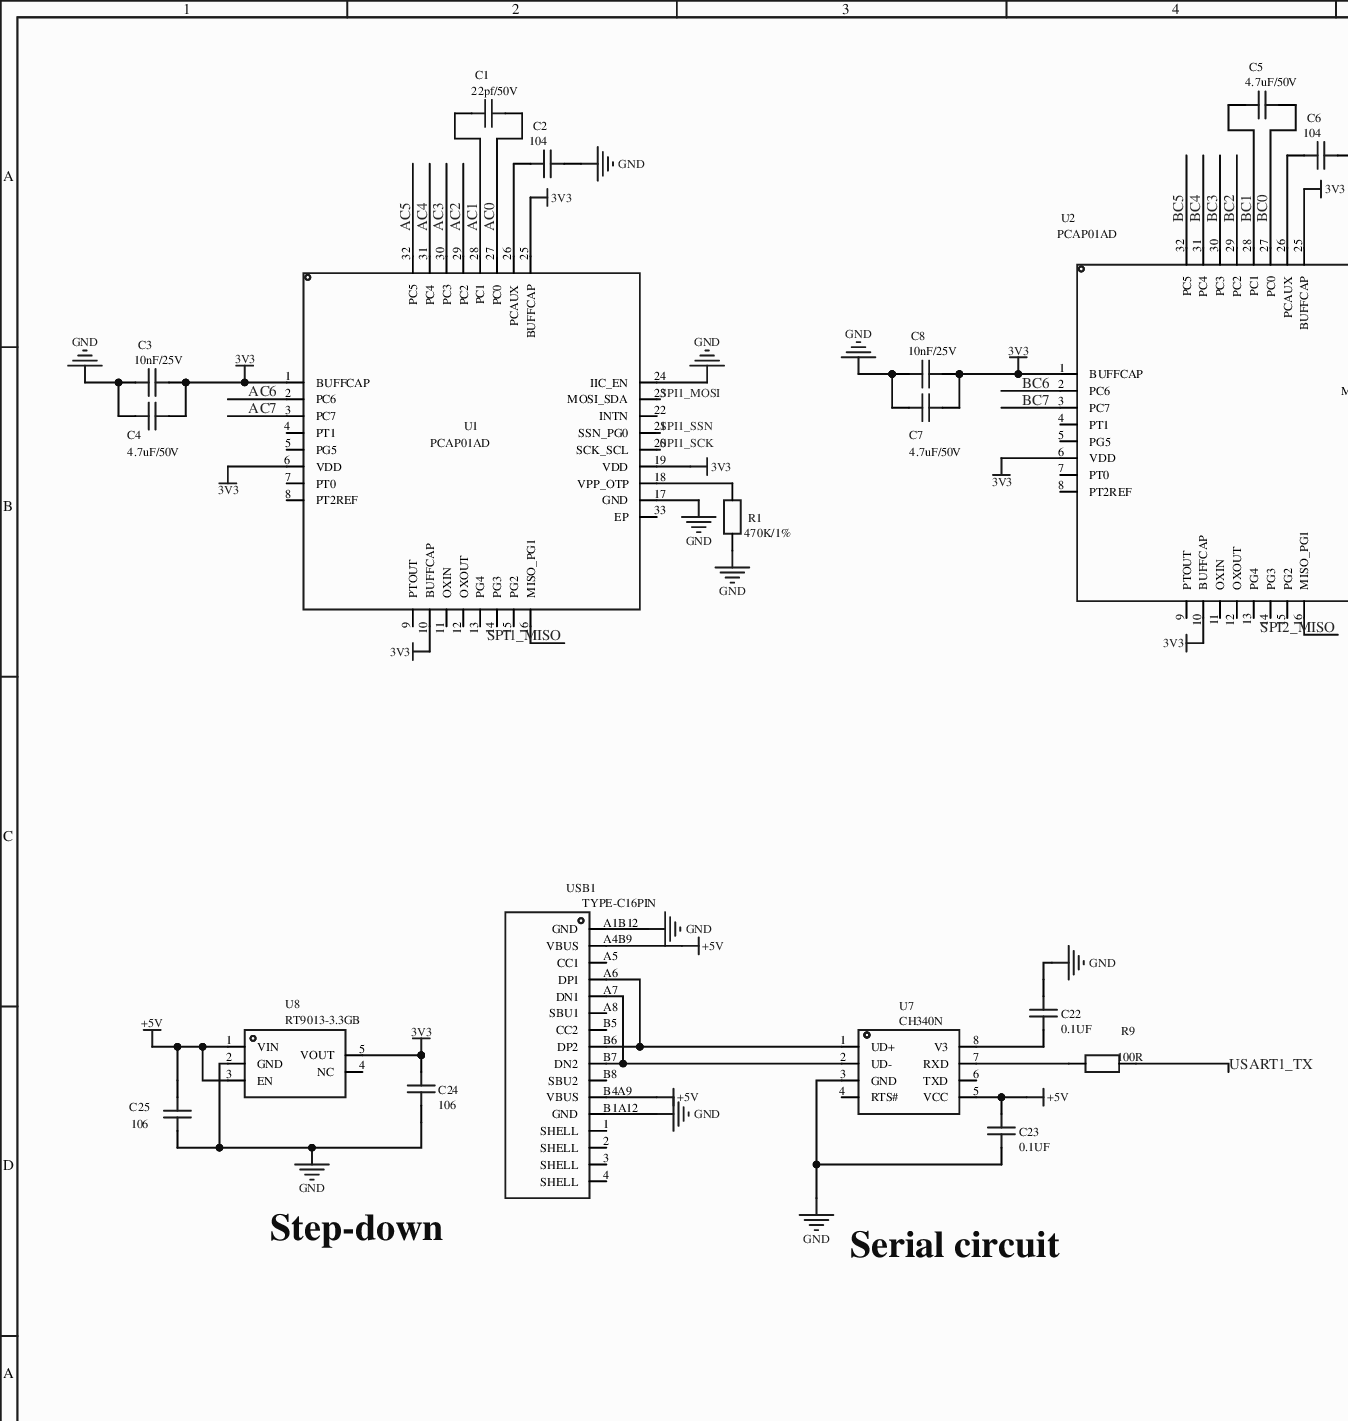
[diagram p0: MISC49858-3.schdoc, top left]
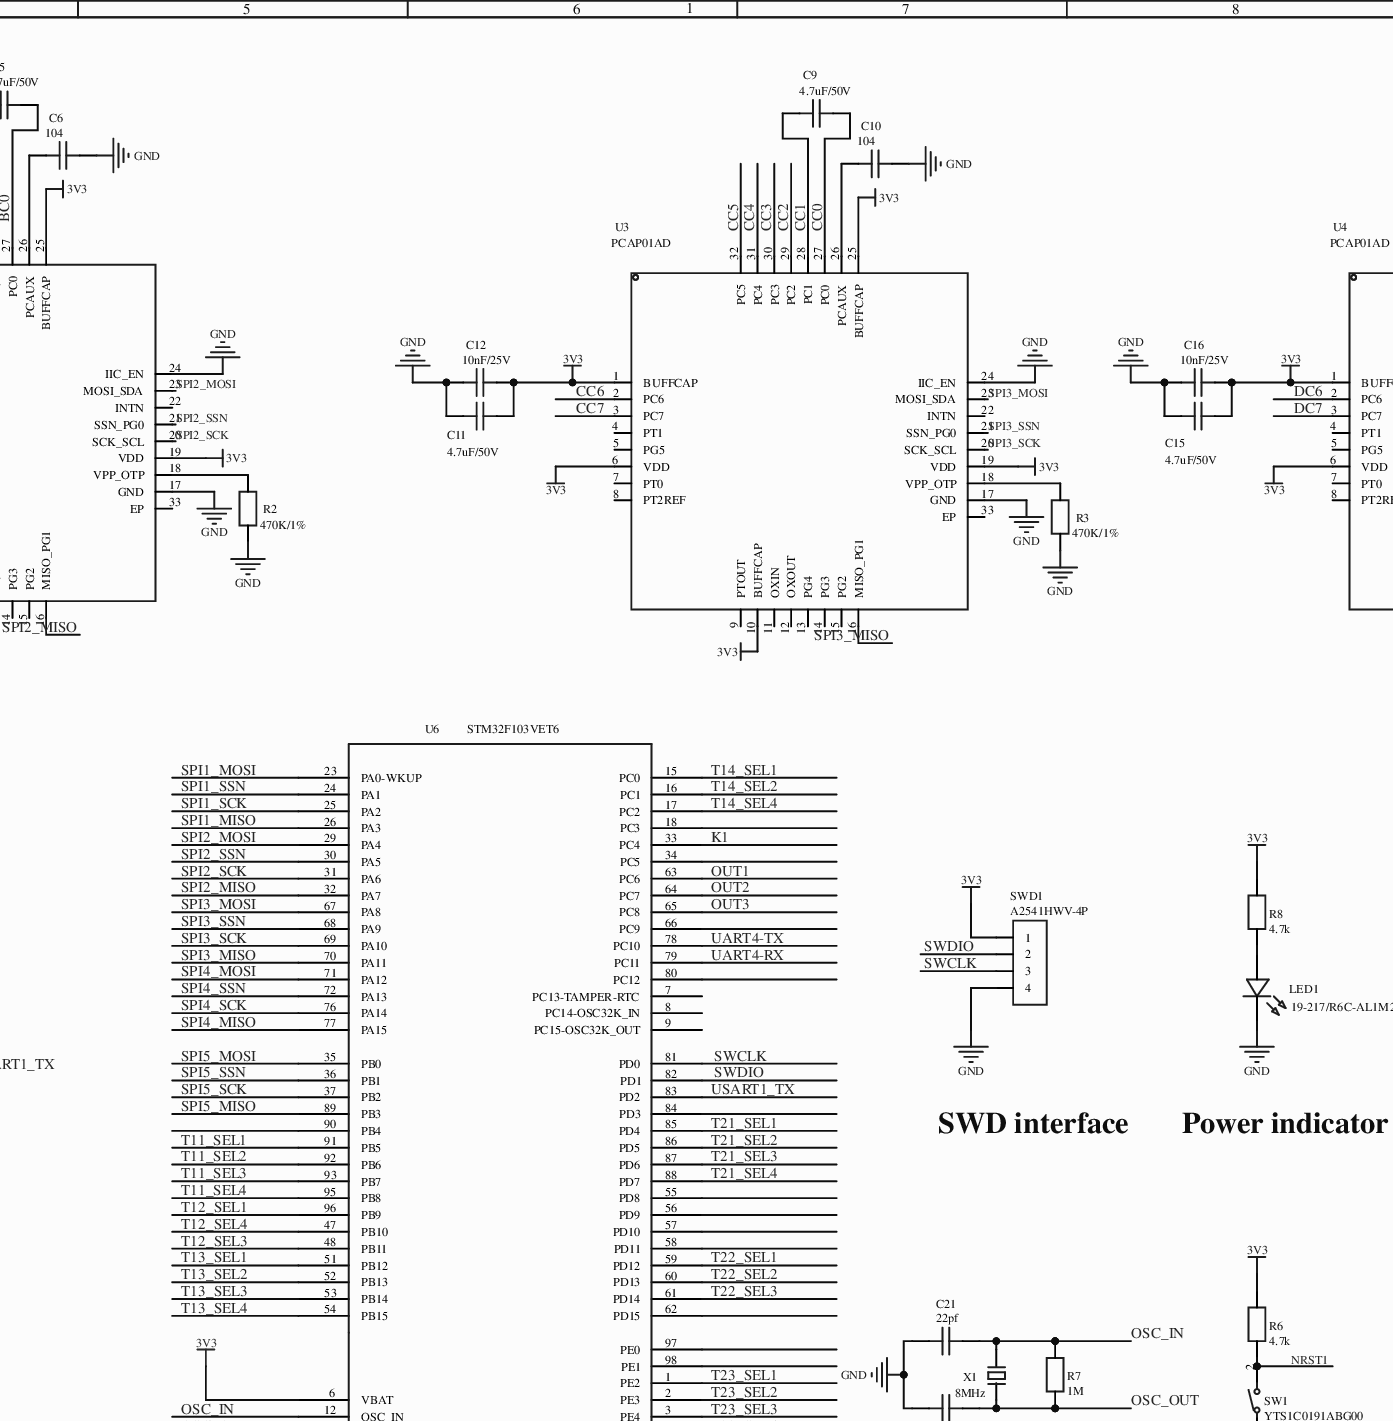
[diagram p1: MISC49858-3.schdoc, top middle]
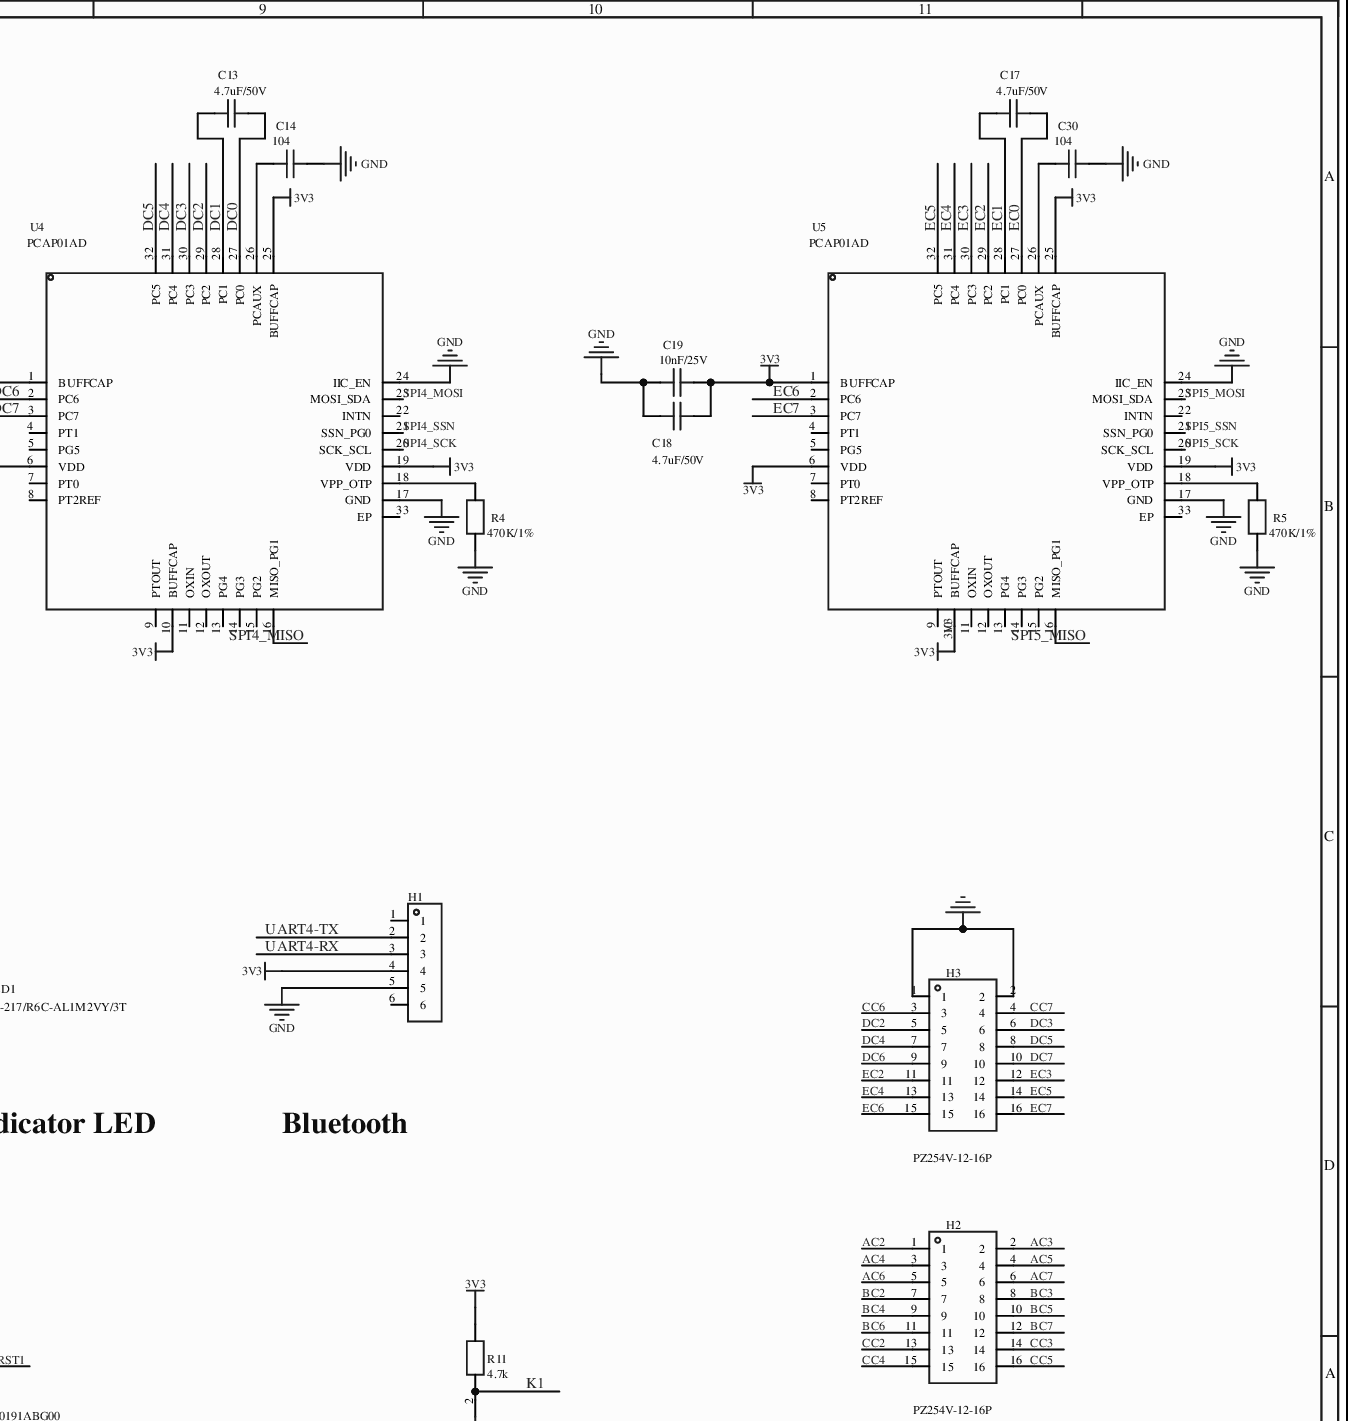
[diagram p2: MISC49858-3.schdoc, top right]
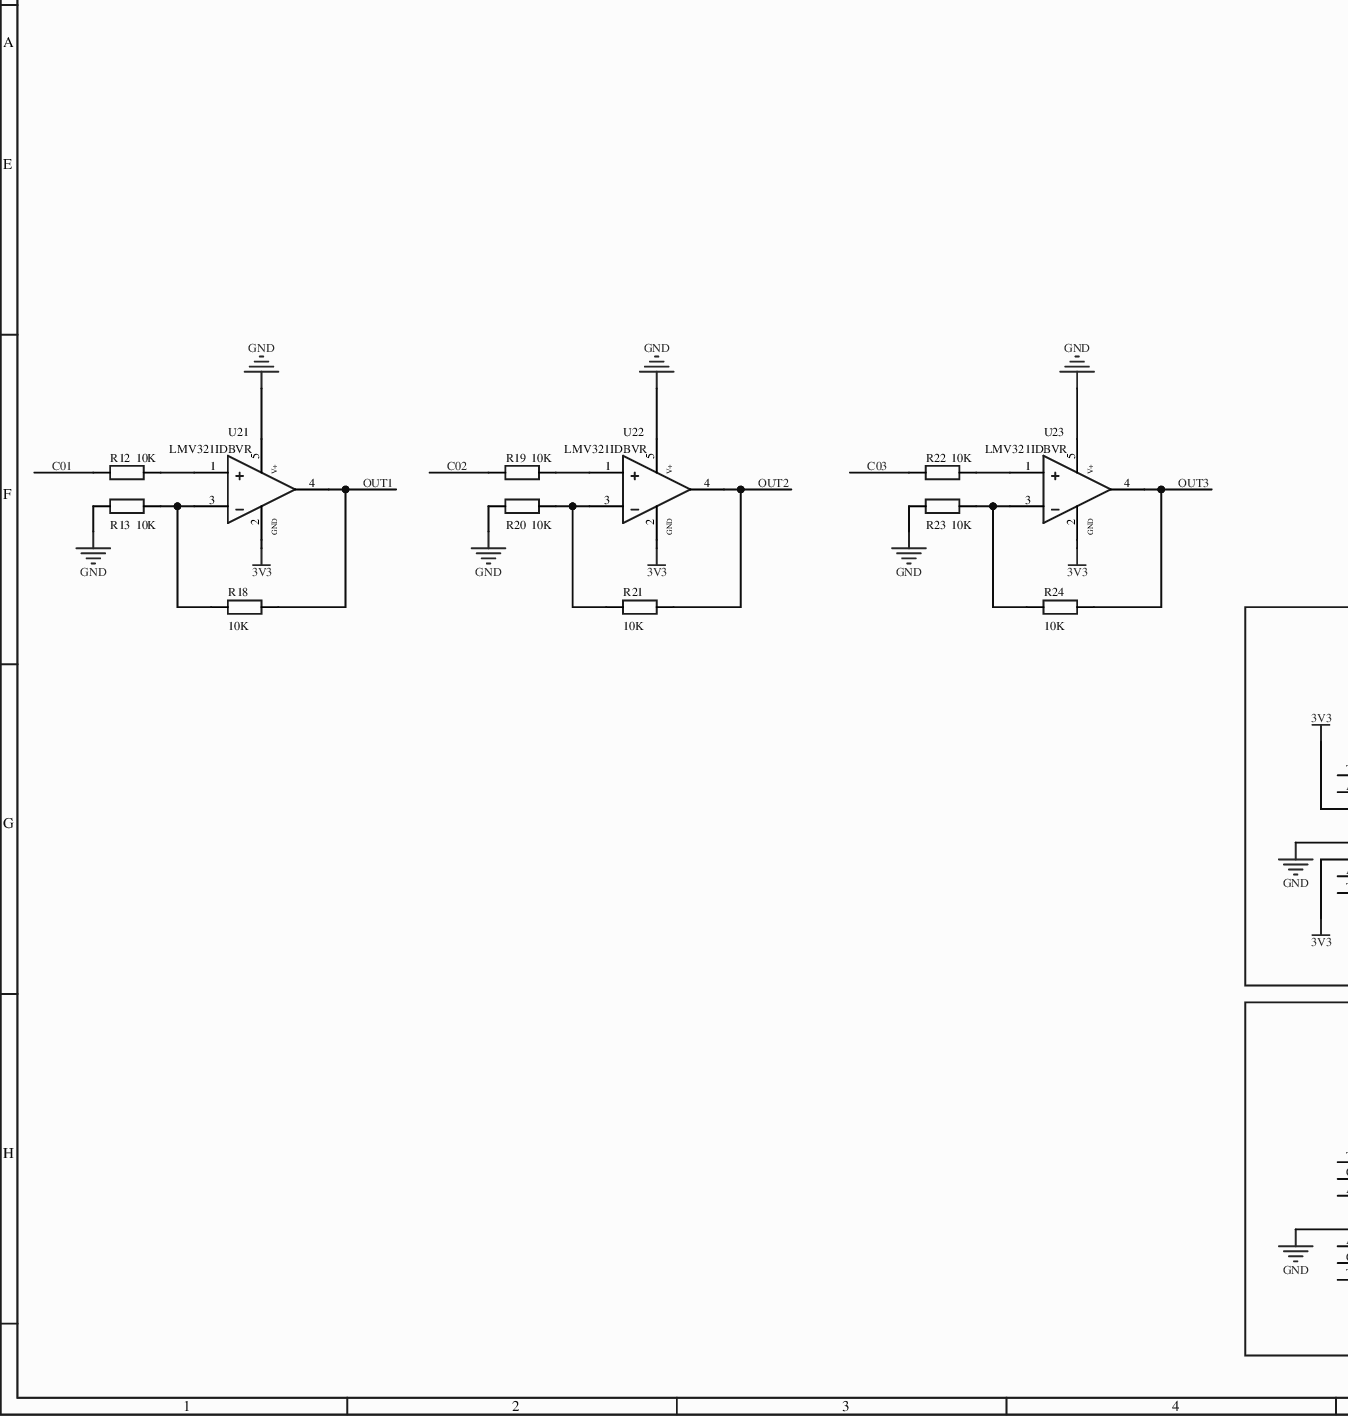
[diagram p3: MISC49858-3.schdoc, bottom left]
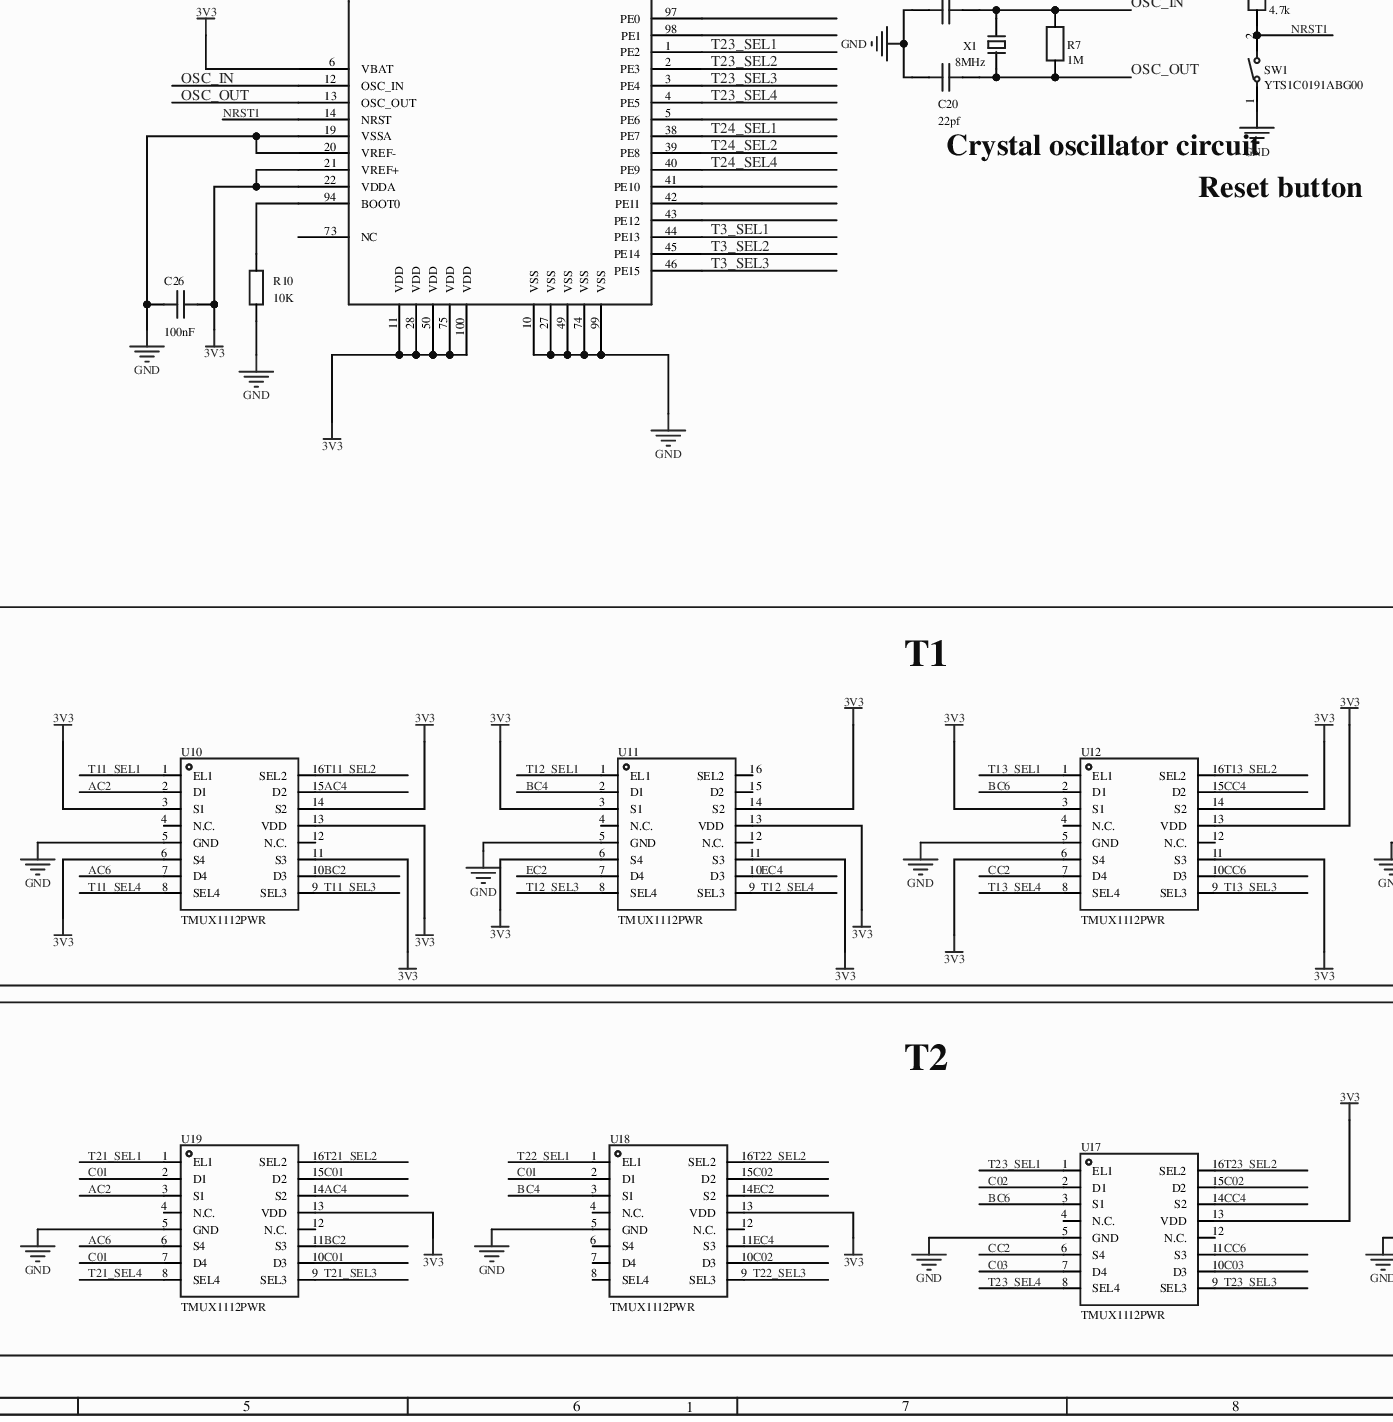
[diagram p4: MISC49858-3.schdoc, bottom middle]
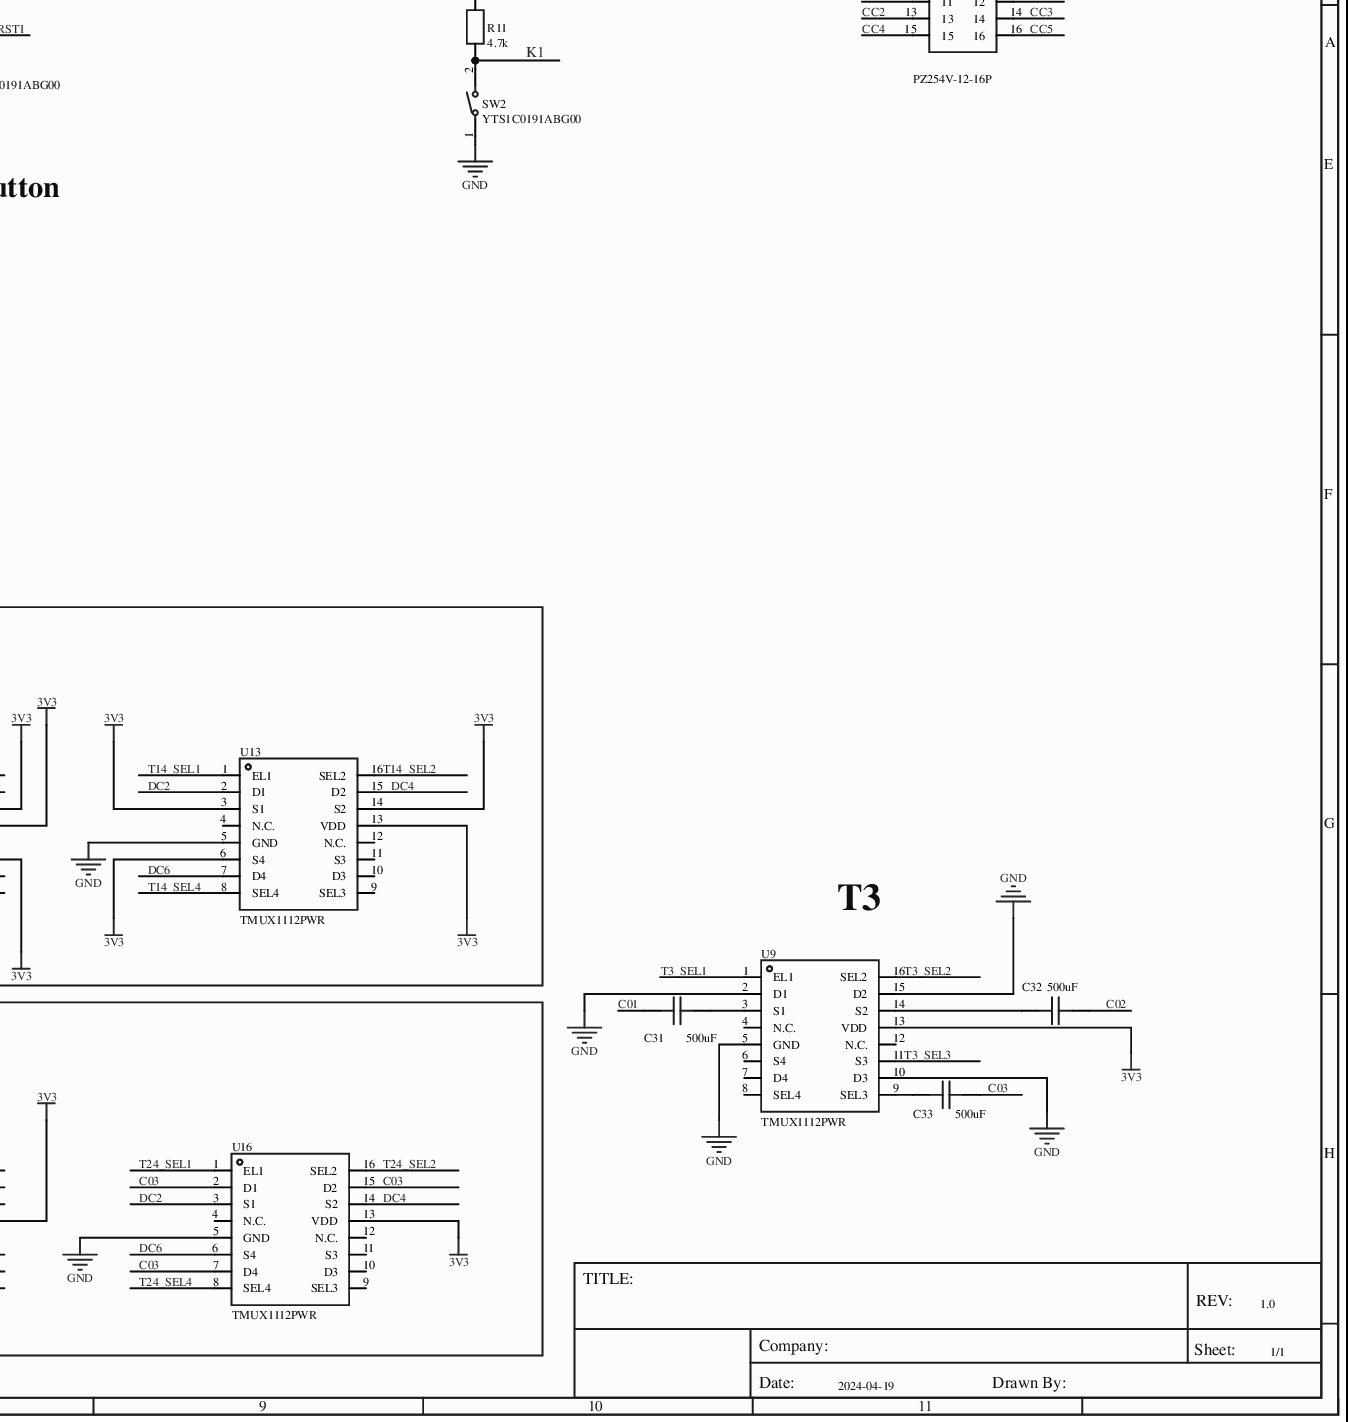
[diagram p5: MISC49858-3.schdoc, bottom right]
# Altium project MISC49858-2.PrjPcb
1 sheet, 79 parts. Net scope: global (net labels, ports and power ports of the same name join across sheets).
Board file: MISC49858.pcbdoc

## Sheet MISC49858-3.schdoc
size 589 x 414 mm; Name: MISC49858; @Project Name: MISC49858; REV: 1.0; Date: 2024-04-19; Sheet: 1/1

### Parts
C1  22pf/50V  [C0603]
C2  104  [C0603]
C3  10nF/25V  [C0603]
C4  4.7uF/50V  [C0603]
C5  4.7uF/50V  [C0603]
C6  104  [C0603]
C7  4.7uF/50V  [C0603]
C8  10nF/25V  [C0603]
C9  4.7uF/50V  [C0603]
C10  104  [C0603]
C11  4.7uF/50V  [C0603]
C12  10nF/25V  [C0603]
C13  4.7uF/50V  [C0603]
C14  104  [C0603]
C15  4.7uF/50V  [C0603]
C16  10nF/25V  [C0603]
C17  4.7uF/50V  [C0603]
C18  4.7uF/50V  [C0603]
C19  10nF/25V  [C0603]
C20  22pf  [C0603]
C21  22pf  [C0603]
C22  0.1UF  [C0603]
C23  0.1UF  [C0603]
C24  106  [C0603]
C25  106  [C0603]
C26  100nF  [C0603]
C30  104  [C0603]
C31  500uF  [C0603]
C32  500uF  [C0603]
C33  500uF  [C0603]
H1  (no value)  [HDR-TH_6P-P2.54-V-F]
H2  PZ254V-12-16P  [HDR-TH_16P-P2.54-V-M-R2-C8-S2.54]
H3  PZ254V-12-16P  [HDR-TH_16P-P2.54-V-M-R2-C8-S2.54]
LED1  19-217/R6C-AL1M2VY/3T  [LED0603-RD]
R1  470K/1%  [R0603]
R2  470K/1%  [R0603]
R3  470K/1%  [R0603]
R4  470K/1%  [R0603]
R5  470K/1%  [R0603]
R6  4.7k  [R0603]
R7  1M  [R0603]
R8  4.7k  [R0603]
R9  100R  [R0603]
R10  10K  [R0603]
R11  4.7k  [R0603]
R12  10K  [R0603]
R13  10K  [R0603]
R18  10K  [R0603]
R19  10K  [R0603]
R20  10K  [R0603]
R21  10K  [R0603]
R22  10K  [R0603]
R23  10K  [R0603]
R24  10K  [R0603]
SW1  YTS1C0191ABG00  [SW-SMD_L6.0-W4.0-LS7.2]
SW2  YTS1C0191ABG00  [SW-SMD_L6.0-W4.0-LS7.2]
SWD1  A2541HWV-4P  [HDR-TH_4P-P2.54-V_A2541HWV-4P]
U1  PCAP01AD  [VQFN-32_L5.0-W5.0-P0.50-TL-EP]
U2  PCAP01AD  [VQFN-32_L5.0-W5.0-P0.50-TL-EP]
U3  PCAP01AD  [VQFN-32_L5.0-W5.0-P0.50-TL-EP]
U4  PCAP01AD  [VQFN-32_L5.0-W5.0-P0.50-TL-EP]
U5  PCAP01AD  [VQFN-32_L5.0-W5.0-P0.50-TL-EP]
U6  STM32F103VET6  [LQFP-100_L14.0-W14.0-P0.50-LS16.0-BL]
U7  CH340N  [SOP-8_150MIL]
U8  RT9013-3.3GB  [SOT-23-5_L2.9-W1.6-P0.94-LS2.8-BL]
U9  TMUX1112PWR  [TSSOP-16_L5.0-W4.4-P0.65-LS6.4-TL]
U10  TMUX1112PWR  [TSSOP-16_L5.0-W4.4-P0.65-LS6.4-TL]
U11  TMUX1112PWR  [TSSOP-16_L5.0-W4.4-P0.65-LS6.4-TL]
U12  TMUX1112PWR  [TSSOP-16_L5.0-W4.4-P0.65-LS6.4-TL]
U13  TMUX1112PWR  [TSSOP-16_L5.0-W4.4-P0.65-LS6.4-TL]
U16  TMUX1112PWR  [TSSOP-16_L5.0-W4.4-P0.65-LS6.4-TL]
U17  TMUX1112PWR  [TSSOP-16_L5.0-W4.4-P0.65-LS6.4-TL]
U18  TMUX1112PWR  [TSSOP-16_L5.0-W4.4-P0.65-LS6.4-TL]
U19  TMUX1112PWR  [TSSOP-16_L5.0-W4.4-P0.65-LS6.4-TL]
U21  LMV321IDBVR  [SOT-23-5_L3.0-W1.7-P0.95-LS2.8-BR]
U22  LMV321IDBVR  [SOT-23-5_L3.0-W1.7-P0.95-LS2.8-BR]
U23  LMV321IDBVR  [SOT-23-5_L3.0-W1.7-P0.95-LS2.8-BR]
USB1  TYPE-C16PIN  [USB-C-SMD_TYPE-C16PIN]
X1  8MHz  [SMD322522]

### Blocks framed on the sheet
T1: U10-U13
T2: U16-U19

### Nets
3V3: C3.2 C4.2 C7.2 C8.2 C11.2 C12.2 C15.2 C16.2 C18.2 C19.2 C24.2 C26.2 H1.4 R6.2 R8.2 R11.2 SWD1.1 U1.1(BUFFCAP) U1.6(VDD) U1.10(BUFFCAP) U1.19(VDD) U1.25(BUFFCAP) U2.1(BUFFCAP) U2.6(VDD) U2.10(BUFFCAP) U2.19(VDD) U2.25(BUFFCAP) U3.1(BUFFCAP) U3.6(VDD) U3.10(BUFFCAP) U3.19(VDD) U3.25(BUFFCAP) U4.1(BUFFCAP) U4.6(VDD) U4.10(BUFFCAP) U4.19(VDD) U4.25(BUFFCAP) U5.1(BUFFCAP) U5.6(VDD) U5.10(BUFFCAP) U5.19(VDD) U5.25(BUFFCAP) U6.6(VBAT) U6.11(VDD) U6.21(VREF+) U6.22(VDDA) U6.28(VDD) U6.50(VDD) U6.75(VDD) U6.100(VDD) U8.5(VOUT) U9.13(VDD) U10.3(S1) U10.6(S4) U10.11(S3) U10.13(VDD) U10.14(S2) U11.3(S1) U11.6(S4) U11.11(S3) U11.13(VDD) U11.14(S2) U12.3(S1) U12.6(S4) U12.11(S3) U12.13(VDD) U12.14(S2) U13.3(S1) U13.6(S4) U13.13(VDD) U13.14(S2) U16.13(VDD) U17.13(VDD) U18.13(VDD) U19.13(VDD) U21.2(GND) U22.2(GND) U23.2(GND)
+5V: C23.2 C25.2 U7.5(VCC) U8.1(VIN) U8.3(EN) USB1.A4B9(VBUS) USB1.B4A9(VBUS)
GND: C2.2 C3.1 C4.1 C6.2 C7.1 C8.1 C10.2 C11.1 C12.1 C14.2 C15.1 C16.1 C18.1 C19.1 C20.1 C21.1 C22.2 C23.1 C24.1 C25.1 C26.1 C30.2 H1.5 H3.1 H3.2 LED1.2 R1.1 R2.1 R3.1 R4.1 R5.1 R10.2 R13.1 R20.1 R23.1 SW1.1 SW2.1 SWD1.4 U1.17(GND) U1.24(IIC_EN) U2.17(GND) U2.24(IIC_EN) U3.17(GND) U3.24(IIC_EN) U4.17(GND) U4.24(IIC_EN) U5.17(GND) U5.24(IIC_EN) U6.10(VSS) U6.19(VSSA) U6.20(VREF-) U6.27(VSS) U6.49(VSS) U6.74(VSS) U6.99(VSS) U7.3(GND) U8.2(GND) U9.2(D1) U9.5(GND) U9.10(D3) U9.15(D2) U10.5(GND) U11.5(GND) U12.5(GND) U13.5(GND) U16.5(GND) U17.5(GND) U18.5(GND) U19.5(GND) U21.5(V+) U22.5(V+) U23.5(V+) USB1.A1B12(GND) USB1.B1A12(GND)  [also labelled NRST]
AC0: C1.2 U1.27(PC0)
AC1: C1.1 U1.28(PC1)
AC2: H2.1 U1.29(PC2) U10.2(D1) U19.3(S1)
AC3: H2.2 U1.30(PC3)
AC4: H2.3 U1.31(PC4) U10.15(D2) U19.14(S2)
AC5: H2.4 U1.32(PC5)
AC6: H2.5 U1.2(PC6) U10.7(D4) U19.6(S4)
AC7: H2.6 U1.3(PC7)
BC0: C5.2 U2.27(PC0)
BC1: C5.1 U2.28(PC1)
BC2: H2.7 U2.29(PC2) U10.10(D3) U19.11(S3)
BC3: H2.8 U2.30(PC3)
BC4: H2.9 U2.31(PC4) U11.2(D1) U18.3(S1)
BC5: H2.10 U2.32(PC5)
BC6: H2.11 U2.2(PC6) U12.2(D1) U17.3(S1)
BC7: H2.12 U2.3(PC7)
C01: C31.2 R12.1 U18.2(D1) U19.2(D1) U19.7(D4) U19.10(D3) U19.15(D2)
C02: C32.1 R19.1 U17.2(D1) U17.15(D2) U18.10(D3) U18.15(D2)
C03: C33.1 R22.1 U16.2(D1) U16.7(D4) U16.15(D2) U17.7(D4) U17.10(D3)
CC0: C9.2 U3.27(PC0)
CC1: C9.1 U3.28(PC1)
CC2: H2.13 U3.29(PC2) U12.7(D4) U17.6(S4)
CC3: H2.14 U3.30(PC3)
CC4: H2.15 U3.31(PC4) U12.15(D2) U17.14(S2)
CC5: H2.16 U3.32(PC5)
CC6: H3.3 U3.2(PC6) U12.10(D3) U17.11(S3)
CC7: H3.4 U3.3(PC7)
DC0: C13.2 U4.27(PC0)
DC1: C13.1 U4.28(PC1)
DC2: H3.5 U4.29(PC2) U13.2(D1) U16.3(S1)
DC3: H3.6 U4.30(PC3)
DC4: H3.7 U4.31(PC4) U13.15(D2) U16.14(S2)
DC5: H3.8 U4.32(PC5)
DC6: H3.9 U4.2(PC6) U13.7(D4) U16.6(S4)
DC7: H3.10 U4.3(PC7)
EC0: C17.2 U5.27(PC0)
EC1: C17.1 U5.28(PC1)
EC2: H3.11 U5.29(PC2) U11.7(D4) U18.14(S2)
EC3: H3.12 U5.30(PC3)
EC4: H3.13 U5.31(PC4) U11.10(D3) U18.11(S3)
EC5: H3.14 U5.32(PC5)
EC6: H3.15 U5.2(PC6)
EC7: H3.16 U5.3(PC7)
K1: R11.1 SW2.2 U6.33(PC4)
NRST1: R6.1 SW1.2 U6.14(NRST)
OSC_IN: C21.2 R7.2 U6.12(OSC_IN) X1.2
OSC_OUT: C20.2 R7.1 U6.13(OSC_OUT) X1.1
OUT1: R18.2 U6.63(PC6) U21.4(OUT)
OUT2: R21.2 U6.64(PC7) U22.4(OUT)
OUT3: R24.2 U6.65(PC8) U23.4(OUT)
SPI1_MISO: U1.16(MISO_PG1) U6.26(PA3)
SPI1_MOSI: U1.23(MOSI_SDA) U6.23(PA0-WKUP)
SPI1_SCK: U1.20(SCK_SCL) U6.25(PA2)
SPI1_SSN: U1.21(SSN_PG0) U6.24(PA1)
SPI2_MISO: U2.16(MISO_PG1) U6.32(PA7)
SPI2_MOSI: U2.23(MOSI_SDA) U6.29(PA4)
SPI2_SCK: U2.20(SCK_SCL) U6.31(PA6)
SPI2_SSN: U2.21(SSN_PG0) U6.30(PA5)
SPI3_MISO: U3.16(MISO_PG1) U6.70(PA11)
SPI3_MOSI: U3.23(MOSI_SDA) U6.67(PA8)
SPI3_SCK: U3.20(SCK_SCL) U6.69(PA10)
SPI3_SSN: U3.21(SSN_PG0) U6.68(PA9)
SPI4_MISO: U4.16(MISO_PG1) U6.77(PA15)
SPI4_MOSI: U4.23(MOSI_SDA) U6.71(PA12)
SPI4_SCK: U4.20(SCK_SCL) U6.76(PA14)
SPI4_SSN: U4.21(SSN_PG0) U6.72(PA13)
SPI5_MISO: U5.16(MISO_PG1) U6.89(PB3)
SPI5_MOSI: U5.23(MOSI_SDA) U6.35(PB0)
SPI5_SCK: U5.20(SCK_SCL) U6.37(PB2)
SPI5_SSN: U5.21(SSN_PG0) U6.36(PB1)
SWCLK: SWD1.3 U6.81(PD0)
SWDIO: SWD1.2 U6.82(PD1)
T3_SEL1: U6.44(PE13) U9.1(EL1)
T3_SEL2: U6.45(PE14) U9.16(SEL2)
T3_SEL3: U6.46(PE15) U9.11(S3)
T11_SEL1: U6.91(PB5) U10.1(EL1)
T11_SEL2: U6.92(PB6) U10.16(SEL2)
T11_SEL3: U6.93(PB7) U10.9(SEL3)
T11_SEL4: U6.95(PB8) U10.8(SEL4)
T12_SEL1: U6.96(PB9) U11.1(EL1)
T12_SEL3: U6.48(PB11) U11.8(SEL4)
T12_SEL4: U6.47(PB10) U11.9(SEL3)
T13_SEL1: U6.51(PB12) U12.1(EL1)
T13_SEL2: U6.52(PB13) U12.16(SEL2)
T13_SEL3: U6.53(PB14) U12.9(SEL3)
T13_SEL4: U6.54(PB15) U12.8(SEL4)
T14_SEL1: U6.15(PC0) U13.1(EL1)
T14_SEL2: U6.16(PC1) U13.16(SEL2)
T14_SEL4: U6.17(PC2) U13.8(SEL4)
T21_SEL1: U6.85(PD4) U19.1(EL1)
T21_SEL2: U6.86(PD5) U19.16(SEL2)
T21_SEL3: U6.87(PD6) U19.9(SEL3)
T21_SEL4: U6.88(PD7) U19.8(SEL4)
T22_SEL1: U6.59(PD12) U18.1(EL1)
T22_SEL2: U6.60(PD13) U18.16(SEL2)
T22_SEL3: U6.61(PD14) U18.9(SEL3)
T23_SEL1: U6.1(PE2) U17.1(EL1)
T23_SEL2: U6.2(PE3) U17.16(SEL2)
T23_SEL3: U6.3(PE4) U17.9(SEL3)
T23_SEL4: U6.4(PE5) U17.8(SEL4)
T24_SEL1: U6.38(PE7) U16.1(EL1)
T24_SEL2: U6.39(PE8) U16.16(SEL2)
T24_SEL4: U6.40(PE9) U16.8(SEL4)
UART4-RX: H1.3 U6.79(PC11)
UART4-TX: H1.2 U6.78(PC10)
USART1_TX: R9.2 U6.83(PD2)
NetC2_1: C2.1 U1.26(PCAUX)
NetC6_1: C6.1 U2.26(PCAUX)
NetC10_1: C10.1 U3.26(PCAUX)
NetC14_1: C14.1 U4.26(PCAUX)
NetC22_1: C22.1 U7.8(V3)
NetC30_1: C30.1 U5.26(PCAUX)
NetC31_1: C31.1 U9.3(S1)
NetC32_2: C32.2 U9.14(S2)
NetC33_2: C33.2 U9.9(SEL3)
NetLED1_1: LED1.1 R8.1
NetR1_2: R1.2 U1.18(VPP_OTP)
NetR2_2: R2.2 U2.18(VPP_OTP)
NetR3_2: R3.2 U3.18(VPP_OTP)
NetR4_2: R4.2 U4.18(VPP_OTP)
NetR5_2: R5.2 U5.18(VPP_OTP)
NetR9_1: R9.1 U7.7(RXD)
NetR10_1: R10.1 U6.94(BOOT0)
NetR12_2: R12.2 U21.1(+)
NetR13_2: R13.2 R18.1 U21.3(-)
NetR19_2: R19.2 U22.1(+)
NetR20_2: R20.2 R21.1 U22.3(-)
NetR22_2: R22.2 U23.1(+)
NetR23_2: R23.2 R24.1 U23.3(-)
NetU7_1: U7.1(UD+) USB1.A6(DP1) USB1.B6(DP2)
NetU7_2: U7.2(UD-) USB1.A7(DN1) USB1.B7(DN2)

Not connected (* = marked no-connect by the designer): H1 1 6; U1 4(PT1)* 5(PG5)* 7(PT0)* 8(PT2REF)* 9(PTOUT)* 11(OXIN)* 12(OXOUT)* 13(PG4)* 14(PG3)* 15(PG2)* 22(INTN)* 33(EP)*; U2 4(PT1)* 5(PG5)* 7(PT0)* 8(PT2REF)* 9(PTOUT)* 11(OXIN)* 12(OXOUT)* 13(PG4)* 14(PG3)* 15(PG2)* 22(INTN)* 33(EP)*; U3 4(PT1)* 5(PG5)* 7(PT0)* 8(PT2REF)* 9(PTOUT)* 11(OXIN)* 12(OXOUT)* 13(PG4)* 14(PG3)* 15(PG2)* 22(INTN)* 33(EP)*; U4 4(PT1)* 5(PG5)* 7(PT0)* 8(PT2REF)* 9(PTOUT)* 11(OXIN)* 12(OXOUT)* 13(PG4)* 14(PG3)* 15(PG2)* 22(INTN)* 33(EP)*; U5 4(PT1)* 5(PG5)* 7(PT0)* 8(PT2REF)* 9(PTOUT)* 11(OXIN)* 12(OXOUT)* 13(PG4)* 14(PG3)* 15(PG2)* 22(INTN)* 33(EP)*; U6 5(PE6) 7(PC13-TAMPER-RTC)* 8(PC14-OSC32K_IN)* 9(PC15-OSC32K_OUT)* 18(PC3) 34(PC5) 41(PE10) 42(PE11) 43(PE12) 55(PD8) 56(PD9) 57(PD10) 58(PD11) 62(PD15) 66(PC9) 73(NC)* 80(PC12) 84(PD3) 90(PB4) 97(PE0) 98(PE1); U7 4(RTS#)* 6(TXD)*; U8 4(NC)*; U9 4(N.C.)* 6(S4)* 7(D4)* 8(SEL4)* 12(N.C.)*; U10 4(N.C.)* 12(N.C.)*; U11 4(N.C.)* 12(N.C.)* 15(D2)* 16(SEL2)*; U12 4(N.C.)* 12(N.C.)*; U13 4(N.C.)* 9(SEL3)* 10(D3)* 11(S3)* 12(N.C.)*; U16 4(N.C.)* 9(SEL3)* 10(D3)* 11(S3)* 12(N.C.)*; U17 4(N.C.)* 12(N.C.)*; U18 4(N.C.)* 6(S4)* 7(D4)* 8(SEL4)* 12(N.C.)*; U19 4(N.C.)* 12(N.C.)*; USB1 1(SHELL)* 2(SHELL)* 3(SHELL)* 4(SHELL)* A5(CC1)* A8(SBU1)* B5(CC2)* B8(SBU2)*

### Notes on the sheet
- SWD interface
- Power indicator LED
- Bluetooth
- Step-down
- Serial circuit
- Crystal oscillator circuit
- Reset button
- (near U9) T3
- 1
- 2
- 3
- 4
- 5
- 6
- 7
- 8
- 9
- 10
- 11
- A
- B
- C
- D
- E
- F
- G
- H
- TITLE:
- Company:
- Sheet:
- REV:
- 1.0
- 1/1
- Date:
- 2024-04-19
- Drawn By:

### Library data of the parts
C1 C4 C5 C7 C9 C11 C13 C15 C17 C18 = 4.7uF/50V: Convert to PCB: yes; 3DModel: C0603_L1.6-W0.8-H0.8; ModelId: fca5be93b99f4b5a9a2fd372d58c31d9; ModelTransform: 0,0,0,0,0,0,0,0,0; Device: 4.7uF/50V; Origin Footprint: C0603; Add into BOM: yes; FootprintName: C0603; ModelName: C0603
  C1: Symbol: 22pf/50V
  C4 C5 C7 C9 C11 C13 C15 C17 C18: Symbol: 4.7uF/50V
C2 C6 C10 C14 C30 = 104: Convert to PCB: yes; 3DModel: C0603_L1.6-W0.8-H0.8; ModelId: fca5be93b99f4b5a9a2fd372d58c31d9; ModelTransform: 0,0,0,0,0,0,0,0,0; Device: 104; Symbol: 104; Origin Footprint: C0603; Add into BOM: yes; FootprintName: C0603; ModelName: C0603
C3 C8 C12 C16 C19 = 10nF/25V: Convert to PCB: yes; 3DModel: C0603_L1.6-W0.8-H0.8; ModelId: fca5be93b99f4b5a9a2fd372d58c31d9; ModelTransform: 0,0,0,0,0,0,0,0,0; Device: 10nF/25V; Symbol: 10nF/25V; Origin Footprint: C0603; Add into BOM: yes; FootprintName: C0603; ModelName: C0603
C20 C21 = 22pf: Convert to PCB: yes; 3DModel: C0603_L1.6-W0.8-H0.8; ModelId: fca5be93b99f4b5a9a2fd372d58c31d9; ModelTransform: 0,0,0,0,0,0,0,0,0; Device: 22pf; Symbol: 22pf; Origin Footprint: C0603; Add into BOM: yes; FootprintName: C0603; ModelName: C0603
C22 C23 = 0.1UF: Convert to PCB: yes; 3DModel: C0603_L1.6-W0.8-H0.8; ModelId: fca5be93b99f4b5a9a2fd372d58c31d9; ModelTransform: 0,0,0,0,0,0,0,0,0; Device: 0.1UF; Symbol: 0.1UF; Origin Footprint: C0603; Add into BOM: yes; FootprintName: C0603; ModelName: C0603
C24 C25 = 106: Convert to PCB: yes; 3DModel: C0603_L1.6-W0.8-H0.8; ModelId: fca5be93b99f4b5a9a2fd372d58c31d9; ModelTransform: 0,0,0,0,0,0,0,0,0; Device: 106; Symbol: 106; Origin Footprint: C0603; Add into BOM: yes; FootprintName: C0603; ModelName: C0603
C26 C31-C33 = CAP_0603: Symbol: Capacitance; ConvertToPcb: yes; ModelId: ac125912035d415993ca9572d50418b1; ModelName: C0603_L1.6-W0.8-H0.8; ModelTransform: 62.992,31.496,0,0,0,0,0,0,0; Device: CAP_0603; FootprintName: C0603; AddInBom: yes; Supplier Footprint: 0603
  C26: Value: 100nF
  C31-C33: Value: 500uF
H1 = HDR-F_2.54_1x6P: Symbol: Header-Female-2.54_1x6; ConvertToPcb: yes; ModelId: 0f5bcf94dcda47d085f24cdca1696fe90819f05c4eef4c71ace90d822a990e87; ModelTransform: 619.684,94.488,0,0,0,0,0,0,-125.984; Device: HDR-F_2.54_1x6P; AddInBom: yes; SupplierPart: C40877; Supplier Footprint: 插件; FootprintName: HDR-TH_6P-P2.54-V-F; ModelName: HDR-TH_6P-P2.54-V-F
H2 H3 = PZ254V-12-16P: Pin structure:2x8P;Pitch:2.54mm;Row spacing:2.54mm;Round/square pin:Square pin;Mounting:Through-hole;Number of rows:Double row;Total pin count:16P;Rated current:-;Rated voltage:-;Mating pin length:6mm;Shell height:2.5mm;Tail pin length:3mm;Contact material:Brass;Contact plating:-;Operating temperature:-40℃~+105℃;Color:Black;; Manufacturer: XFCN(兴飞); AddInBom: yes; Pin Structure: 2x8P; Pitch: 2.54mm; ModelId: 4229ed04564d49dfa51d40f734d422b6; ModelName: HDR2.54-M-LI-2X8P; ModelTransform: 799.99844,200,0,0,0,0,0,0,-118.11; Device: PZ254V-12-16P; Symbol: PZ254V-12-16P; FootprintName: HDR-TH_16P-P2.54-V-M-R2-C8-S2.54; LCSC Part Name: 2x8P 间距:2.54mm 方针 直插; SupplierPart: C492425; ManufacturerPart: PZ254V-12-16P; Supplier Footprint: 插件,P=2.54mm; JLCPCB Part Class: Extended Part; Datasheet: example.com/datasheet/PZ254V-12-16P/502981.html; Supplier: LCSC; ConvertToPcb: yes; Row Spacing: 2.54mm; Circluar Pins/Square Pins: Square pin; Mounting Type: Through-hole; Number of Rows: Double row; Number of Pins: 16P; Current Rating: -; Voltage Rating (Max): -; Length of Mating Pin: 6mm; Insulation Height: 2.5mm; Length of End Connection Pin: 3mm; Contact Material: Brass; Contact Plating: -; Operating Temperature: -40℃~+105℃; Color: Black
LED1 = 19-217/R6C-AL1M2VY/3T: Illumination color:Red;Forward voltage (Vf):1.95V;Power:60mW;Forward current:5mA;Wavelength:617.5nm;Diode configuration:-;Lens color:Colorless transparent lens;Color temperature:-;Viewing angle:120°;Tape packaging:-;Operating temperature:-40℃~+85℃;; Manufacturer: EVERLIGHT(亿光); Symbol: LED-0603_R; 3DModel: LED0603_Red; Convert to PCB: yes; Illumination Color: Red; Voltage - Forward(Vf): 1.95V; Power(Watts): 60mW; Forward Current: 5mA; Peak Wavelength: 632nm; Viewing Angle: 120°; ModelId: 1f0d29a91be547639d425604e9b96ebb; ModelTransform: 63.7794,32.283,0,0,0,0,0,0,0; Device: 19-217/R6C-AL1M2VY/3T; Origin Footprint: LED0603_RED; Manufacturer Part: 19-217/R6C-AL1M2VY/3T; Supplier Part: C72044; Supplier: LCSC; Add into BOM: yes; FootprintName: LED0603-RD; LCSC Part Name: 红灯 停产; Supplier Footprint: 0603; JLCPCB Part Class: Extended Part; Wavelength - Dominant: 617.5nm; Diode Configuration: -; Lens Color: Colorless transparent lens; Color Temperature: -; Mounting Style: -; Operating Temperature: -40℃~+85℃; ModelName: LED0603-RD
R1-R5 = 470K/1%: Convert to PCB: yes; ModelId: fc143cca1e79419f9cd78b61e9279f08; ModelTransform: 0,0,0,0,0,0,0,0,0; Device: 470K/1%; Symbol: 470K/1%; Origin Footprint: R0603; Add into BOM: yes; FootprintName: R0603; 3DModel: R0603; link: example.com/datasheet/2/447/PYu_RT_1_to_0_01_RoHS_L_11-1669912.pdf; ModelName: R0603
R6 R8 R11 = 4.7k: Convert to PCB: yes; ModelId: fc143cca1e79419f9cd78b61e9279f08; ModelTransform: 0,0,0,0,0,0,0,0,0; Device: 4.7k; Symbol: 4.7k; Origin Footprint: R0603; Add into BOM: yes; FootprintName: R0603; 3DModel: R0603; link: example.com/datasheet/2/447/PYu_RT_1_to_0_01_RoHS_L_11-1669912.pdf; ModelName: R0603
R7 = 1M: Convert to PCB: yes; ModelId: fc143cca1e79419f9cd78b61e9279f08; ModelTransform: 0,0,0,0,0,0,0,0,0; Device: 1M; Symbol: 1M; Origin Footprint: R0603; Add into BOM: yes; FootprintName: R0603; 3DModel: R0603; link: example.com/datasheet/2/447/PYu_RT_1_to_0_01_RoHS_L_11-1669912.pdf; ModelName: R0603
R9 = 100R: Convert to PCB: yes; ModelId: fc143cca1e79419f9cd78b61e9279f08; ModelTransform: 0,0,0,0,0,0,0,0,0; Device: 100R; Symbol: 100R; Origin Footprint: R0603; Add into BOM: yes; FootprintName: R0603; 3DModel: R0603; link: example.com/datasheet/2/447/PYu_RT_1_to_0_01_RoHS_L_11-1669912.pdf; ModelName: R0603
R10 = Res_0603: Symbol: Resistor; ConvertToPcb: yes; ModelId: fc143cca1e79419f9cd78b61e9279f08; ModelTransform: 0,0,0,0,0,0,0,0,0; Device: Res_0603; Value: 10K; FootprintName: R0603; AddInBom: yes; Supplier Footprint: 0603; ModelName: R0603
R12 R13 R18-R24 = Res_0603: Symbol: Resistor; 3D Model: fc143cca1e79419f9cd78b61e9279f08; 3D Model Transform: 31.8897,63.7794,0,90,0,0,0,0,0; ConvertToPcb: yes; Device: Res_0603; Supplier Footprint: 0603; Value: 10K; FootprintName: R0603; AddInBom: yes; ModelName: R0603
SW1 SW2 = YTS1C0191ABG00: Manufacturer: YIYUAN(怡远); Convert to PCB: yes; ModelId: 849019bbab9849c7984437acb3e659b5; ModelTransform: 0,0,0,0,0,0,0,0,0; Device: YTS1C0191ABG00; Symbol: YTS1C0191ABG00; Origin Footprint: SW-SMD_L6.0-W4.0-LS7.2; Supplier: LCSC; Supplier Part: C2985764; Manufacturer Part: YTS1C0191ABG00; link: example.com/upload/public/pdf/source/20220324/CA2613BFC4B8BE6894B6D74C5E7CD5F6.pdf; JLCPCB Part Class: Extended Part; Add into BOM: yes; FootprintName: SW-SMD_L6.0-W4.0-LS7.2; 3DModel: SW-SMD_L6.0-W4.0-LS7.2; ModelName: SW-SMD_L6.0-W4.0-LS7.2
SWD1 = A2541HWV-4P: Socket structure:1x4P;Pitch:2.54mm;Row spacing:-;Round/square hole:Square hole;Mounting:Through-hole;Number of rows:Single row;Total hole count:4P;Rated current:3A;Rated voltage:250V;Socket direction:Top;Shell height:8.5mm;Contact material:Brass;Contact plating:Gold;Operating temperature:-40℃~+105℃;; Manufacturer: CJT(长江连接器); Symbol: HDR-F-2.54_1x4; Convert to PCB: yes; Holes Structure: 1x4P; Pitch: 2.54mm; Number of Positions: 4P; Current Rating: 3A; Voltage Rating (Max): 250V; Holes Direction: Top; PIN Length: 3.2mm; ModelId: 4a7f96097dcd477d8f9da3e104374928; ModelTransform: 399.999,100,0,0,0,0,0,0,-118.11; Device: A2541HWV-4P; 3DModel: HDR-F-2.54_1x4; Origin Footprint: HDR-F-2.54_1X4; Supplier Part: C225501; Supplier: LCSC; Manufacturer Part: A2541HWV-4P; Add into BOM: yes; FootprintName: HDR-TH_4P-P2.54-V_A2541HWV-4P; LCSC Part Name: 1x4P 间距:2.54mm 直插; Supplier Footprint: 插件,P=2.54mm; JLCPCB Part Class: Extended Part; Datasheet: example.com/datasheet/A2541HWV-4P/225784.html; Row Spacing: -; Circular Hole / Square Hole: Square hole; Mounting Type: Through-hole; Number of Rows: Single row; Insulation Height: 8.5mm; Contact Material: Brass; Contact Plating: Gold; Operating Temperature: -40℃~+105℃; ModelName: HDR-F-2.54_1x4
U1-U5 = PCAP01AD: Resolution:17-bit;Operating voltage:2.1V~3.6V;Interface type:SPI; I2C;; Manufacturer: Sciosense; 3DModel: VQFN-32_L5.0-W5.0-H1.0-P0.50; Convert to PCB: yes; Resolution(Bits): 17-bit; number of channels: 8; ModelId: 9b1a95a4ec4749e3b92af9df887435c6; ModelTransform: 197.6374,197.6374,0,0,0,0,-0.0005,0,0; Device: PCAP01AD; Symbol: PCAP01AD; Origin Footprint: VQFN-32_L5.0-W5.0-P0.50-TL-EP; Supplier: LCSC; Supplier Part: C192738; Manufacturer Part: PCAP01AD; JLCPCB Part Class: Extended Part; Add into BOM: yes; FootprintName: VQFN-32_L5.0-W5.0-P0.50-TL-EP; LCSC Part Name: PCAP01AD; Supplier Footprint: QFN-32-EP(5x5); Datasheet: example.com/upload/public/pdf/source/20180601/C192738_90641FB33958A3184578B590A974B57E.pdf; Voltage - Supply: 2.1V~3.6V; Interface: SPI; I2C; differential input: -; Operating Temperature: -40℃~+125℃; ModelName: VQFN-32_L5.0-W5.0-H1.0-P0.50
U6 = STM32F103VET6: CPU core:ARM-M3;Max CPU frequency:72MHz;Application field:-;; Manufacturer: ST(意法半导体); AddInBom: yes; CPU Core: ARM-M3; CPU Maximum Speed: 72MHz; Program Storage Size: 512KB; Program Memory Type: FLASH; Number of I/O: 80; ADC (Bit): 12bit; Voltage - Supply: 2V~3.6V; ModelId: 469e6cc70557486dbd01fd12ff814964; ModelName: LQFP-100_L14.0-W14.0-H1.4-LS16.0-P0.50; ModelTransform: 629.92,629.92,0,0,0,0,0,0,0; Device: STM32F103VET6; Symbol: STM32F103VET6; FootprintName: LQFP-100_L14.0-W14.0-P0.50-LS16.0-BL; LCSC Part Name: 主流增强型ARM Cortex-M3 MCU，具有512 KB Flash、72 MHz CPU、电机控制、USB和CAN; SupplierPart: C8308; ManufacturerPart: STM32F103VET6; Supplier Footprint: LQFP-100(14x14); JLCPCB Part Class: Extended Part; Datasheet: example.com/datasheet/STM32F103VET6/8800.html; Supplier: LCSC; ConvertToPcb: yes; DAC (Bit): 12bit; Applications: -
U7 = CH340N: Manufacturer: WCH; Convert to PCB: yes; ModelId: 556e10306cd14ddf90ed6175cd2ed7f3; ModelTransform: 0,0,0,0,0,0,0,0,0; Device: CH340N; Symbol: CH340N; Origin Footprint: SOP-8_150MIL; Manufacturer Part: CH340N; Add into BOM: yes; FootprintName: SOP-8_150MIL; ModelName: SOP-8_150MIL
U8 = RT9013-3.3GB: Manufacturer: null; Convert to PCB: yes; ModelId: 842a9d81c16647a78bb4654fd7d034e5; ModelTransform: 114.173,110.236,0,0,0,0,0,0,0; Device: RT9013-3.3GB; Symbol: RT9013-3.3GB; link: example.com/datasheet-pdf/view/304739/POWER/LP4062-B5F.html; 3DModel: SOT-23-5_L2.9-W1.6-P0.94-LS2.8-BL; Origin Footprint: SOT-23-5_L2.9-W1.6-P0.94-LS2.8-BL; Supplier: LCSC; Supplier Part: C9900009203; Manufacturer Part: RT9013-3.3GB; JLCPCB Part Class: Extended Part; Add into BOM: yes; FootprintName: SOT-23-5_L2.9-W1.6-P0.94-LS2.8-BL; LCSC Part Name: RT9013-3.3GB; Supplier Footprint: SOT-23-5; ModelName: SOT-23-5_L2.9-W1.6-P0.94-LS2.8-BL
U9-U13 U16-U19 = TMUX1112PWR: Switch circuit:Single-pole single-throw (SPST);Channel count:4;On-resistance (Ron@VCC):4Ω;; Manufacturer: TI(德州仪器); AddInBom: yes; Number of Channels: 4; Supply Voltage: 1.08V~5.5V; On-State Resistance (Max): 4Ω; ModelId: e184b9ae7def452b81228c95a013214c; ModelName: TSSOP-16_L5.0-W4.4-H1.0-LS6.4-P0.65; ModelTransform: 252.188,196.85,0,0,0,0,0,-0.002,0; Device: TMUX1112PWR; Symbol: TMUX1112PWR; FootprintName: TSSOP-16_L5.0-W4.4-P0.65-LS6.4-TL; LCSC Part Name: TMUX111x 5V、低泄漏电流、1:1(SPST)、4通道精密开关; SupplierPart: C2877031; ManufacturerPart: TMUX1112PWR; Supplier Footprint: TSSOP-16; JLCPCB Part Class: Extended Part; Supplier: LCSC; ConvertToPcb: yes; Switch Circuit: Single-pole single-throw (SPST)
U21-U23 = LMV321IDBVR_C7972: Amplifier count:Single;Rail-to-rail:Rail-to-rail output;Gain bandwidth product (GBP):1MHz;Input offset voltage (Vos):7mV;Slew rate (SR):1V/us;Input bias current (Ib):11nA;; Manufacturer: TI(德州仪器); AddInBom: yes; Number of Channels: Single; Maximum Power Supply Range (Vdd-Vss): 5.5V; Gain Bandwidth Product: 1MHz; Vos - Input Offset Voltage: 7mV; Input Offset Voltage Drift(Vos TC): 9uV/℃; Slew Rate: 1V/us; Ib - Input Bias Current: 11nA; Input Offset Current(Ios): 5nA; Noise density(eN): 46nV/√Hz@1kHz; Common Mode Rejection Ratio(CMRR): 63dB; Quiescent Current: 170uA; Output Current: 5mA; Single supply: 2.7V~5.5V; ModelId: 0a2a1b8f50944f73965918ad6e5fe1670819f05c4eef4c71ace90d822a990e87; ModelName: SOT-23-5_L2.9-W1.6-H1.1-LS2.8-P0.95; ModelTransform: 114.173,109.636,0,180,0,0,0,0,0; Device: LMV321IDBVR_C7972; Symbol: LMV321IDBVR; FootprintName: SOT-23-5_L3.0-W1.7-P0.95-LS2.8-BR; LCSC Part Name: 低电压轨到轨输出运算放大器; SupplierPart: C7972; ManufacturerPart: LMV321IDBVR; Supplier Footprint: SOT-23-5; JLCPCB Part Class: Extended Part; Supplier: LCSC; ConvertToPcb: yes; Rail to Rail: Rail-to-rail output; Input offset current drift(Ios TC): -; Operating Temperature: -40℃~+125℃
USB1 = TYPE-C16PIN: Connector type:Type-C;Protocol standard:USB 3.1;Gender:Female;Mounting:Flat-mount;Contact count:16P;Port count:1;Rated current - power:3A;Operating temperature:-40℃~+85℃;; Manufacturer: SHOU HAN(首韩); Origin Footprint: USB-C-SMD_TYPE-C16PIN_C668624; Convert to PCB: yes; Connector Type: Type-C; Protocol Standard: USB 3.1; Gender: Female; Number of Contacts: 16P; Number of Ports: 1; Current Rating-Power: 3A; Voltage Rating: 30V; Connect-Disconnect Life: 1 ten-thousand cycles; Detection color: Black; ModelId: d6783d3a2268456b863f42d3286191d0; ModelTransform: 351.9678,311.023,0,180,0,0,0,-41.85,-39.37; Device: TYPE-C16PIN; Symbol: TYPE-C16PIN; 3DModel: USB-C-SMD_TYPE-C16PIN; Supplier: LCSC; Supplier Part: C393939; Manufacturer Part: TYPE-C16PIN; Add into BOM: yes; FootprintName: USB-C-SMD_TYPE-C16PIN; LCSC Part Name: Type-C 母 卧贴; Supplier Footprint: SMD; JLCPCB Part Class: Extended Part; Datasheet: example.com/datasheet/TYPE-C16PIN/372551.html; Mounting Type: Flat-mount; Operating Temperature: -40℃~+85℃; ModelName: USB-C-SMD_TYPE-C16PIN
X1 = 8MHz: BOM名称: 2-pin passive crystal oscillator; 版权归属: COMPANY_A; Convert to PCB: yes; Device: 8MHz; Symbol: 8MHz; Origin Footprint: SMD322522; Add into BOM: yes; FootprintName: SMD322522